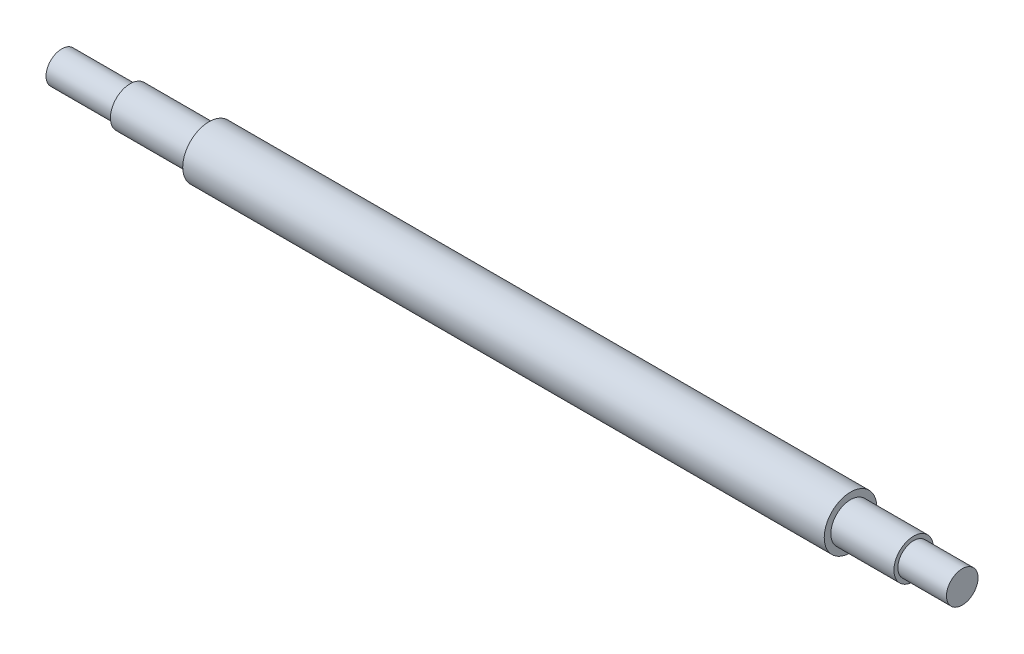
from build123d import *


with BuildPart() as part:
    # 草图1 → 旋转1 (revolve)
    with BuildSketch(Plane.XY, mode=Mode.PRIVATE) as revolve_1_sk:
        Polygon((-94.709677419, 0), (-94.709677419, 12), (-42.709677419, 12), (-42.709677419, 15), (17.290322581, 15), (17.290322581, 20), (505.290322581, 20), (505.290322581, 15), (553.290322581, 15), (553.290322581, 12), (590.290322581, 12), (590.290322581, 0), align=None)
    revolve(revolve_1_sk.sketch.rotate(Axis((-124.903225806, 0, 0), (1, 0, 0)), 90), axis=Axis((-124.903225806, 0, 0), (1, 0, 0)))


solid = part.part
